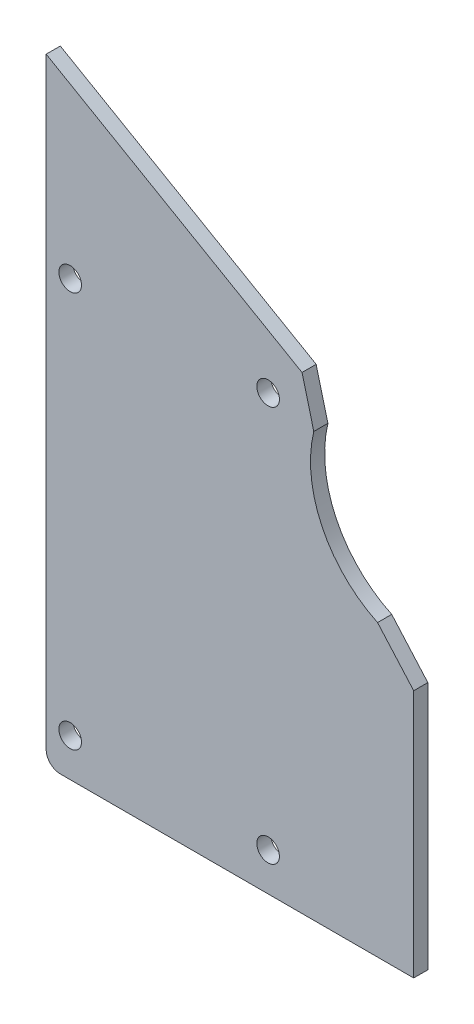
SolidWorks part; units mm, degrees
material "Q235B"
ref_plane "Front Plane" through (0, 0, 0) normal (0, 0, 1) x (1, 0, 0)
ref_plane "Top Plane" through (0, 0, 0) normal (0, 1, 0) x (1, 0, 0)
ref_plane "Right Plane" through (0, 0, 0) normal (1, 0, 0) x (0, 0, -1)
sketch "Sketch1" plane through (0, 0, 0) normal (0, 0, 1) x (1, 0, 0)
  line L0 (0, 0) -> (0, 436)
  line L1 (0, 436) -> (181, 331.4996)
  line L2 (181, 331.4996) -> (189.3231, 299.4996)
  line L3 (0, 0) -> (260, 0)
  line L4 (260, 0) -> (260, 176)
  line L5 (260, 176) -> (234.4472, 205)
  arc A1 (234.4472, 205) -> (189.3231, 299.4996) centre (270, 280) cw
  dimension "D1" = 181
  dimension "D7" = 10
  dimension "D9" = 83
  dimension "D2" = 436
  dimension "D3" = 120
  dimension "D4" = 32
  dimension "D5" = 176
  dimension "D6" = 29
  dimension "D8" = 260
  dimension "D10" = 280
extrude "Boss-Extrude1" add sketch "Sketch1" along normal mid plane 10
hole_wizard "Ø16.0 (16) Diameter Hole1" positions "Sketch2" profile "Sketch3" hole size "Ø16.0" standard "GB" end condition up to next
sketch "Sketch2" plane through (0, 0, 5) normal (0, 0, 1) x (1, 0, 0)
  line L0 (17, 27) -> (157, 27) construction
  line L1 (17, 27) -> (17, 307) construction
  line L2 (260, 0) -> (260, 176) construction
  line L3 (0, 0) -> (260, 0) construction
  point P0 (17, 27)
  point P6 (157, 27)
  point P7 (157, 307)
  point P8 (17, 307)
  dimension "D3" = 90
  dimension "D4" = 140
  dimension "D5" = 280
  dimension "D6" = 103
  dimension "D7" = 27
  dimension "D1" = 2
  dimension "D2" = 2
sketch "Sketch3" plane through (17, 27, 5) normal (1, 0, 0) x (0, -1, 0)
  line L0 (0, 0) -> (0, 10)
  line L1 (0, 10) -> (8, 10)
  line L2 (8, 10) -> (8, 0)
  line L5 (8, 0) -> (0, 0)
  line L11 (0, -6.35) -> (0, 107.95) construction
  dimension "通孔孔直径" = 16
  dimension "通孔孔深度" = 10
fillet "Fillet1" radius 10 1 edges at (0, 0, 0)
